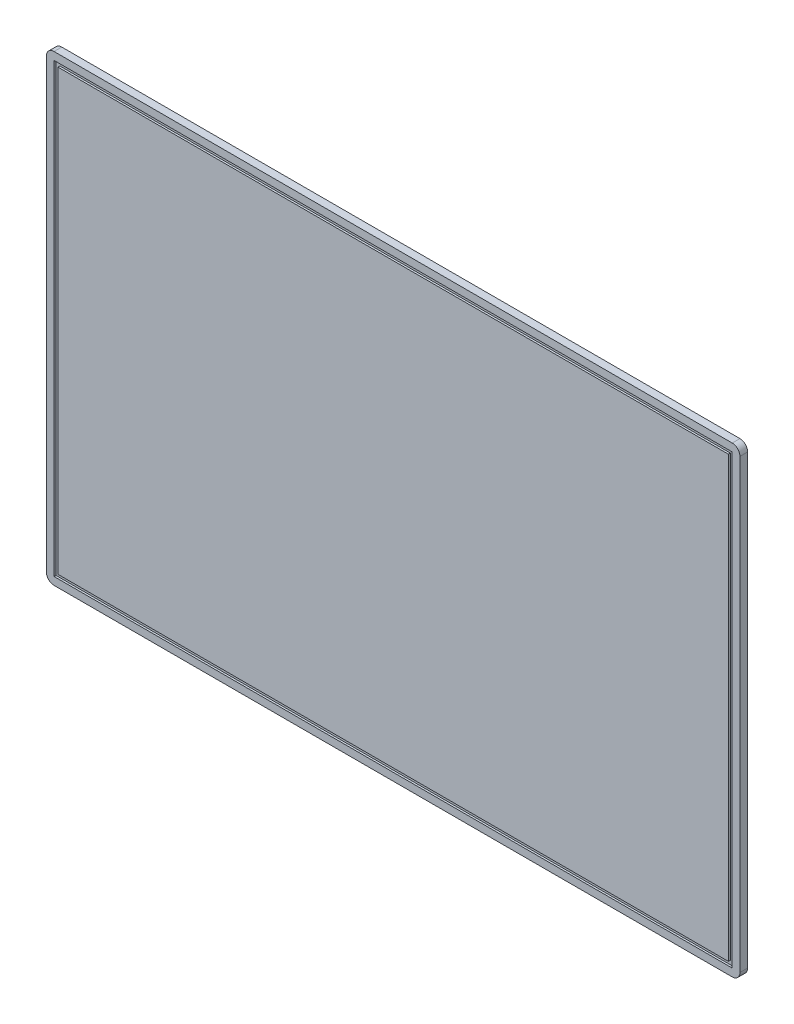
from build123d import *

# Parameters (mm, degrees)
BOSS_EXTRUDE1_DEPTH = 2
SKETCH2_W           = 176
SKETCH2_H           = 116
SKETCH2_W_2         = 174
SKETCH2_H_2         = 114
CUT_EXTRUDE1_DEPTH  = 0.5


with BuildPart() as part:
    # Sketch1 → Boss-Extrude1 (new body)
    with BuildSketch(Plane.XY):
        with BuildLine():
            Line((88, 60), (-88, 60))
            ThreePointArc((-88, 60), (-89.414213562, 59.414213562), (-90, 58))
            Line((-90, 58), (-90, -58))
            ThreePointArc((-90, -58), (-89.414213562, -59.414213562), (-88, -60))
            Line((-88, -60), (88, -60))
            ThreePointArc((88, -60), (89.414213562, -59.414213562), (90, -58))
            Line((90, -58), (90, 58))
            ThreePointArc((90, 58), (89.414213562, 59.414213562), (88, 60))
        make_face()
    extrude(amount=BOSS_EXTRUDE1_DEPTH)

    # Sketch2 → Cut-Extrude1 (cut)
    with BuildSketch(Plane.XY.offset(2)):
        Rectangle(SKETCH2_W, SKETCH2_H)
        Rectangle(SKETCH2_W_2, SKETCH2_H_2, mode=Mode.SUBTRACT)
    extrude(amount=-CUT_EXTRUDE1_DEPTH, mode=Mode.SUBTRACT)


solid = part.part
